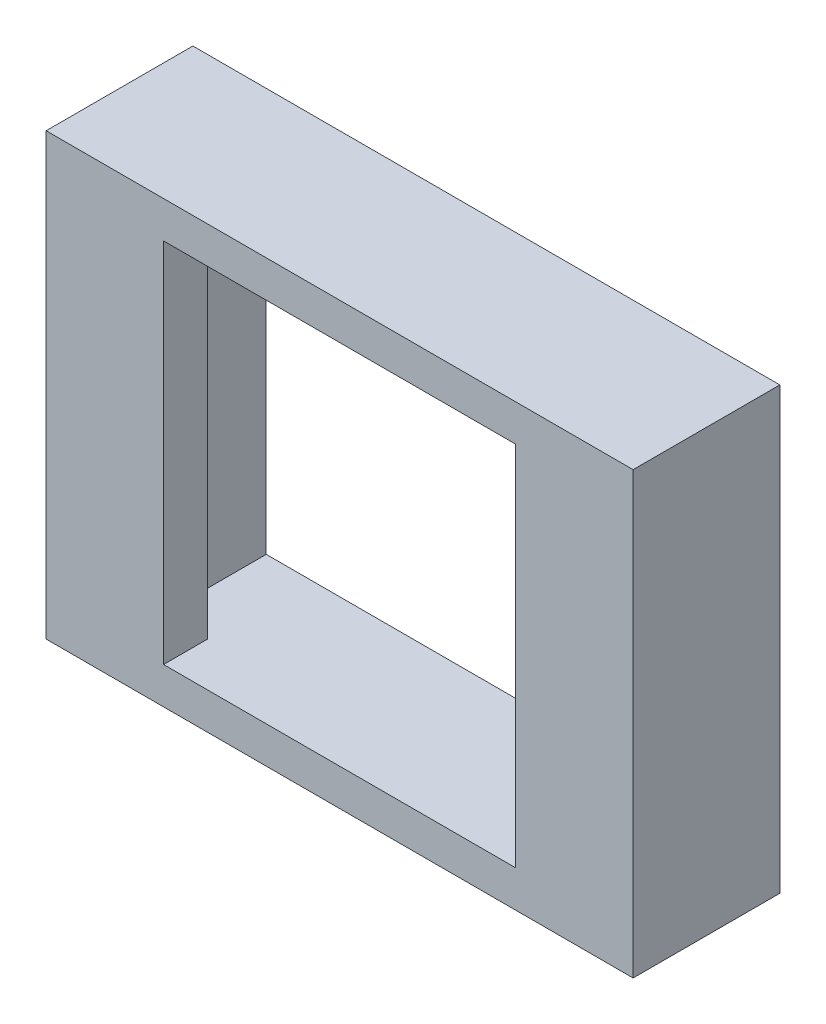
SolidWorks part; units mm, degrees
material "45"
ref_plane "前视基准面" through (0, 0, 0) normal (0, 0, 1) x (1, 0, 0)
ref_plane "上视基准面" through (0, 0, 0) normal (0, 1, 0) x (1, 0, 0)
ref_plane "右视基准面" through (0, 0, 0) normal (1, 0, 0) x (0, 0, -1)
sketch "草图1" plane through (0, 0, 0) normal (0, 0, 1) x (1, 0, 0)
  line L1 (40, -30) -> (-40, -30)
  line L2 (40, -30) -> (40, 30)
  line L3 (40, 30) -> (-40, 30)
  line L4 (-40, -30) -> (-40, 30)
  line L5 (40, -30) -> (-40, 30) construction
  line L6 (40, 30) -> (-40, -30) construction
  point P0 (0, 0)
  dimension "D1" = 80
  dimension "D2" = 60
extrude "凸台-拉伸1" add sketch "草图1" along normal blind 20
sketch "草图2" plane through (0, 0, 20) normal (0, 0, 1) x (1, 0, 0)
  line L1 (24, -25) -> (-24, -25)
  line L2 (24, -25) -> (24, 25)
  line L3 (24, 25) -> (-24, 25)
  line L4 (-24, -25) -> (-24, 25)
  line L5 (24, -25) -> (-24, 25) construction
  line L6 (24, 25) -> (-24, -25) construction
  point P0 (0, 0)
  dimension "D1" = 50
  dimension "D2" = 48
extrude "切除-拉伸1" cut sketch "草图2" against normal up to next
sketch "草图3" plane through (0, 0, 0) normal (0, 0, -1) x (-1, 0, 0)
  line L0 (24, 25) -> (-24, 25) construction
  line L1 (30, -25) -> (-30, -25)
  line L2 (30, -25) -> (30, 25)
  line L3 (30, 25) -> (-30, 25)
  line L4 (-30, -25) -> (-30, 25)
  line L5 (30, -25) -> (-30, 25) construction
  line L6 (30, 25) -> (-30, -25) construction
  point P0 (0, 0)
  dimension "D1" = 60
extrude "切除-拉伸2" cut sketch "草图3" against normal blind 14
